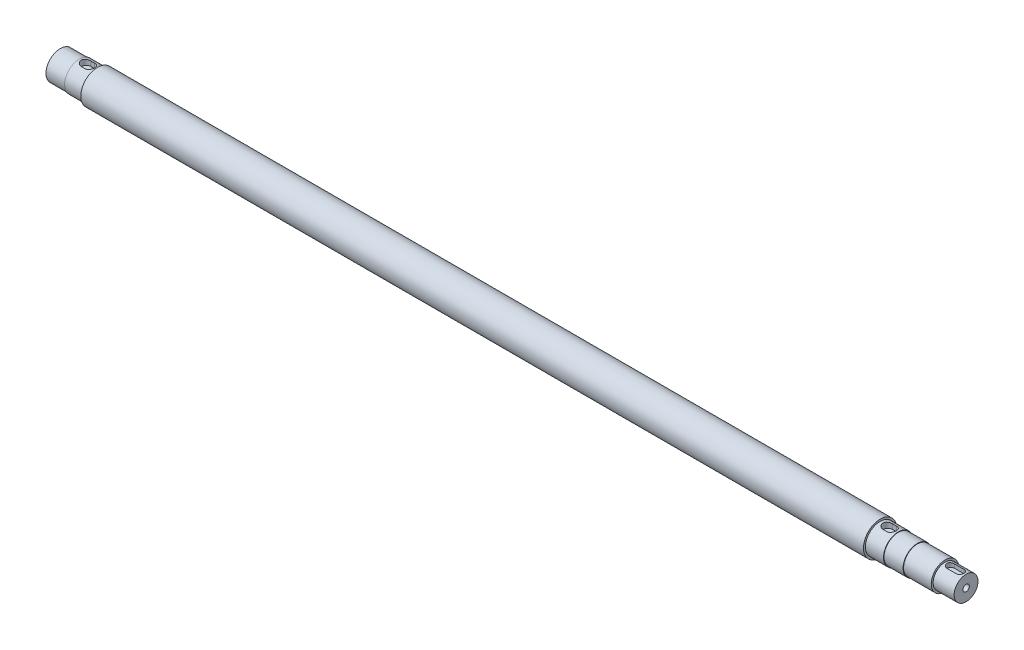
from build123d import *

# Parameters (mm, degrees)
SKETCH_1_R             = 17.5
EXTRUDE_1_DEPTH        = 410
SKETCH_2_R             = 15.5
EXTRUDE_2_DEPTH        = 19
SKETCH_3_R             = 15
EXTRUDE_3_DEPTH        = 20
SKETCH_4_R             = 14.5
EXTRUDE_4_DEPTH        = 29
SKETCH_5_R             = 12.5
EXTRUDE_5_DEPTH        = 22
CUT_EXTRUDE_1_DEPTH    = 5.83
CUT_EXTRUDE_2_DEPTH    = 7.66
HOLE_WIZARD_M8_1_D     = 6.8
HOLE_WIZARD_M8_1_DEPTH = 20
HOLE_WIZARD_M8_1_TIP   = 2.042926105


with BuildPart() as part:
    # 草图1 → 凸台-拉伸1 (new, symmetric)
    with BuildSketch(Plane(origin=(0, 0, 0), x_dir=(0, 0, -1), z_dir=(1, 0, 0))):
        with Locations(Location((0, 0, 0), (0, 0, 180))):
            Circle(SKETCH_1_R)
    extrude(amount=EXTRUDE_1_DEPTH, both=True)

    # 草图2 → 凸台-拉伸2 (add)
    with BuildSketch(Plane(origin=(410, 0, 0), x_dir=(0, 0, -1), z_dir=(1, 0, 0))):
        Circle(SKETCH_2_R)
    extrude_2 = extrude(amount=EXTRUDE_2_DEPTH)

    # 草图3 → 凸台-拉伸3 (add)
    with BuildSketch(Plane(origin=(429, 0, 0), x_dir=(0, 0, -1), z_dir=(1, 0, 0))):
        Circle(SKETCH_3_R)
    extrude_3 = extrude(amount=EXTRUDE_3_DEPTH)

    # 草图4 → 凸台-拉伸4 (add)
    with BuildSketch(Plane(origin=(449, 0, 0), x_dir=(0, 0, -1), z_dir=(1, 0, 0))):
        with Locations(Location((0, 0, 0), (0, 0, 180))):
            Circle(SKETCH_4_R)
    extrude(amount=EXTRUDE_4_DEPTH)

    # 草图5 → 凸台-拉伸5 (add)
    with BuildSketch(Plane(origin=(478, 0, 0), x_dir=(0, 0, -1), z_dir=(1, 0, 0))):
        Circle(SKETCH_5_R)
    extrude(amount=EXTRUDE_5_DEPTH)

    # 镜向1: 凸台-拉伸2, 凸台-拉伸3 across plane
    add(extrude_2.mirror(Plane(origin=(0, 0, 0), x_dir=(0, 0, 1), z_dir=(1, 0, 0))))
    add(extrude_3.mirror(Plane(origin=(0, 0, 0), x_dir=(0, 0, 1), z_dir=(1, 0, 0))))

    # 草图6 → 切除-拉伸1 (cut)
    with BuildSketch(Plane(origin=(0, 15.5, 0), x_dir=(1, 0, 0), z_dir=(0, 1, 0))):
        with BuildLine():
            Line((-418, -5), (-422, -5))
            ThreePointArc((-422, -5), (-427, 0), (-422, 5))
            Line((-422, 5), (-418, 5))
            ThreePointArc((-418, 5), (-413, 0), (-418, -5))
        make_face()
        with BuildLine():
            Line((422, -5), (418, -5))
            ThreePointArc((418, -5), (413, 0), (418, 5))
            Line((418, 5), (422, 5))
            ThreePointArc((422, 5), (427, 0), (422, -5))
        make_face()
    extrude(amount=-CUT_EXTRUDE_1_DEPTH, mode=Mode.SUBTRACT)

    # 草图7 → 切除-拉伸2 (cut)
    with BuildSketch(Plane(origin=(0, 15.5, 0), x_dir=(1, 0, 0), z_dir=(0, 1, 0))):
        with BuildLine():
            Line((484, 4), (494, 4))
            ThreePointArc((494, 4), (498, 0), (494, -4))
            Line((494, -4), (484, -4))
            ThreePointArc((484, -4), (480, 0), (484, 4))
        make_face()
    extrude(amount=-CUT_EXTRUDE_2_DEPTH, mode=Mode.SUBTRACT)

    # M8 螺纹孔1
    with Locations(Plane(origin=(500, 0, 0), x_dir=(0, 0, -1), z_dir=(1, 0, 0))):
        with Locations((0, 0)):
            Hole(HOLE_WIZARD_M8_1_D / 2, depth=HOLE_WIZARD_M8_1_DEPTH)
            with Locations((0, 0, -(HOLE_WIZARD_M8_1_DEPTH + HOLE_WIZARD_M8_1_TIP / 2))):  # 118° drill point
                Cone(0, HOLE_WIZARD_M8_1_D / 2, HOLE_WIZARD_M8_1_TIP, mode=Mode.SUBTRACT)


solid = part.part
